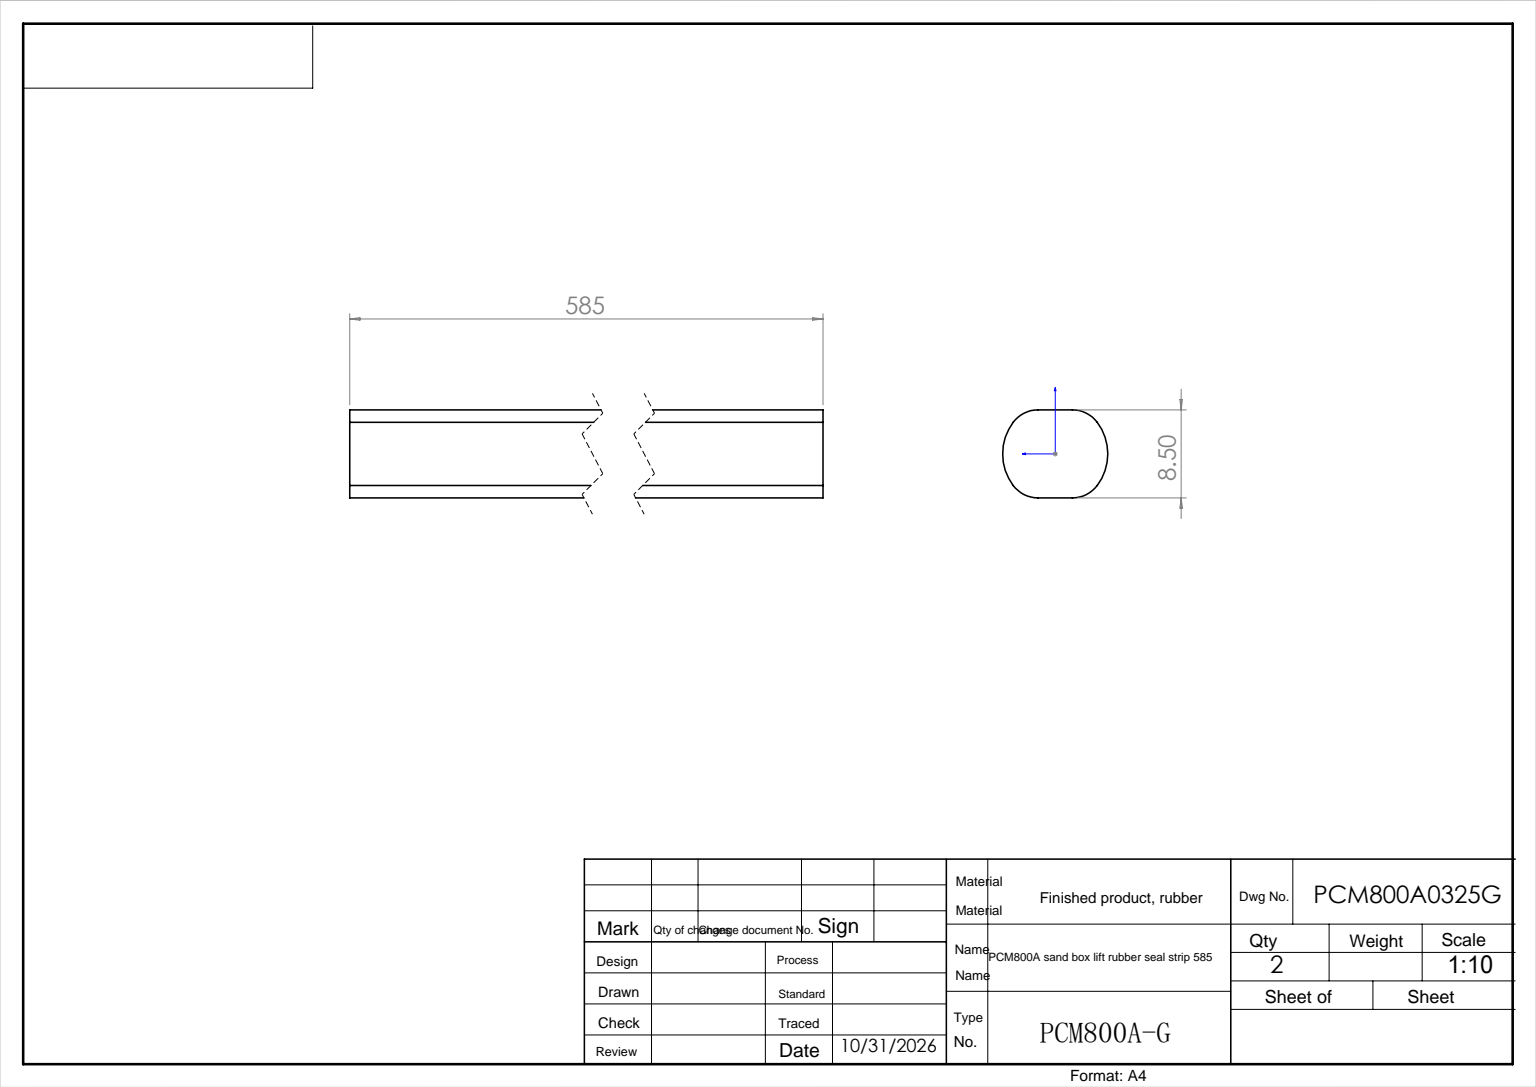
from build123d import *

# Parameters (mm, degrees)
EXTRUDE_1_DEPTH = 585


with BuildPart() as part:
    # 草图1 → 拉伸1 (new body)
    with BuildSketch(Plane.XY):
        with BuildLine():
            Line((-1.661470687, 4.25), (1.661470687, 4.25))
            ThreePointArc((1.661470687, 4.25), (3.001099397, 3.934286669), (4.058769011, 3.053596614))
            ThreePointArc((4.058769011, 3.053596614), (5.079178887, 0), (4.058769011, -3.053596614))
            ThreePointArc((4.058769011, -3.053596614), (3.001099397, -3.934286669), (1.661470687, -4.25))
            Line((1.661470687, -4.25), (-1.661470687, -4.25))
            ThreePointArc((-1.661470687, -4.25), (-3.001099397, -3.934286669), (-4.058769011, -3.053596614))
            ThreePointArc((-4.058769011, -3.053596614), (-5.079178887, 0), (-4.058769011, 3.053596614))
            ThreePointArc((-4.058769011, 3.053596614), (-3.001099397, 3.934286669), (-1.661470687, 4.25))
        make_face()
    extrude(amount=EXTRUDE_1_DEPTH)


solid = part.part
